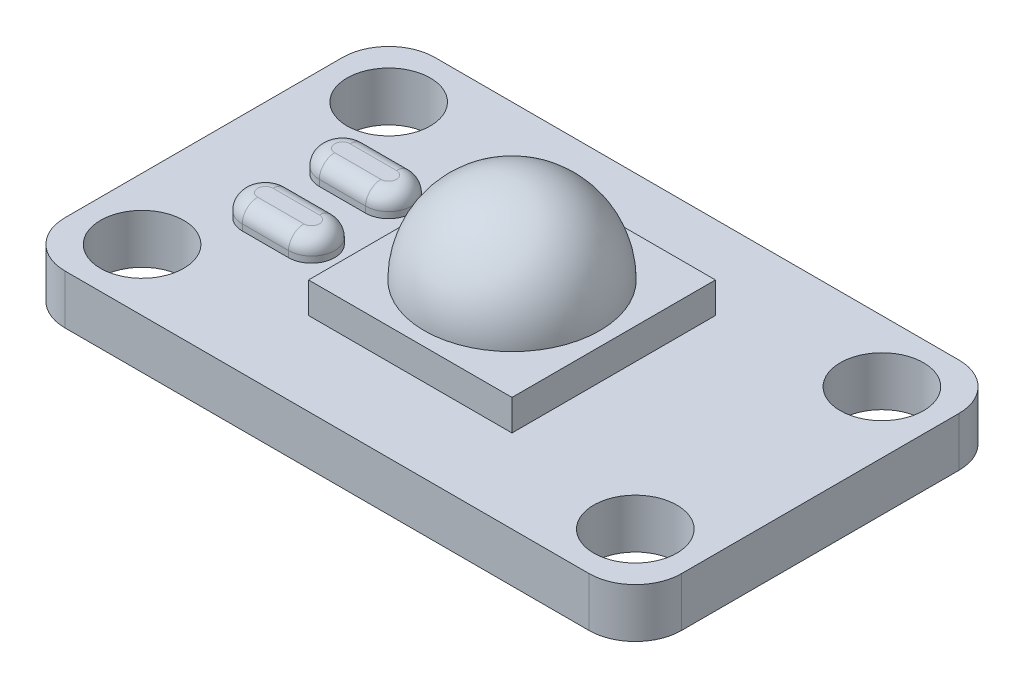
SolidWorks part; units mm, degrees
ref_plane "前视基准面" through (0, 0, 0) normal (0, 0, 1) x (1, 0, 0)
ref_plane "上视基准面" through (0, 0, 0) normal (0, 1, 0) x (1, 0, 0)
ref_plane "右视基准面" through (0, 0, 0) normal (1, 0, 0) x (0, 0, -1)
sketch "铝基板外型" plane through (0, 0, 0) normal (0, 1, 0) x (1, 0, 0)
  line L1 (-8.5, -6) -> (8.5, -6)
  line L2 (-10, -4.5) -> (-10, 4.5)
  line L3 (-8.5, 6) -> (8.5, 6)
  line L4 (10, -4.5) -> (10, 4.5)
  line L5 (-10, -6) -> (10, 6) construction
  line L6 (-10, 6) -> (10, -6) construction
  arc A0 (-8.5, -6) -> (-10, -4.5) centre (-8.5, -4.5) cw
  arc A1 (8.5, -6) -> (10, -4.5) centre (8.5, -4.5) ccw
  arc A2 (8.5, 6) -> (10, 4.5) centre (8.5, 4.5) cw
  arc A3 (-10, 4.5) -> (-8.5, 6) centre (-8.5, 4.5) cw
  point P0 (0, 0)
  dimension "D1" = 1.5
  dimension "D2" = 20
  dimension "D3" = 12
extrude "铝基板" add sketch "铝基板外型" along normal blind 1.6
sketch "草图7" plane through (0, 0, 0) normal (0, 1, 0) x (1, 0, 0)
  line L1 (-8, -4) -> (8, -4) construction
  line L2 (-8, -4) -> (-8, 4) construction
  line L3 (-8, 4) -> (8, 4) construction
  line L4 (8, -4) -> (8, 4) construction
  line L5 (-8, -4) -> (8, 4) construction
  line L6 (-8, 4) -> (8, -4) construction
  circle A0 centre (-8, -4) radius 1.35
  circle A1 centre (8, -4) radius 1.35
  circle A2 centre (8, 4) radius 1.35
  circle A3 centre (-8, 4) radius 1.35
  point P0 (0, 0)
  dimension "D3" = 2.7
  dimension "D1" = 8
  dimension "D2" = 16
extrude "螺丝孔" cut sketch "草图7" along normal through all
sketch "？？？" plane through (0, 1.6, 0) normal (0, 1, 0) x (1, 0, 0)
  line L1 (-3.3, 3.3) -> (3.3, 3.3)
  line L2 (-3.3, 3.3) -> (-3.3, -3.3)
  line L3 (-3.3, -3.3) -> (3.3, -3.3)
  line L4 (3.3, 3.3) -> (3.3, -3.3)
  line L5 (-3.3, 3.3) -> (3.3, -3.3) construction
  line L6 (-3.3, -3.3) -> (3.3, 3.3) construction
  point P0 (0, 0)
  dimension "D1" = 6.6
extrude "灯珠板" add sketch "？？？" along normal blind 1 separate body
sketch "灯珠旋转基础" plane through (0, 0, 0) normal (0, 0, 1) x (1, 0, 0)
  line L0 (0, 2.6) -> (2.85, 2.6)
  line L1 (0, 2.6) -> (0, 5.45)
  line L2 (-3.3, 2.6) -> (3.3, 2.6) construction
  arc A0 (0, 5.45) -> (2.85, 2.6) centre (0, 2.6) cw
  dimension "D1" = 2.85
revolve "灯珠" add sketch "灯珠旋转基础" angle 360 about L1
sketch "焊盘" plane through (0, 1.6, 0) normal (0, 1, 0) x (1, 0, 0)
  line L0 (-6.75, 1.25) -> (-5.25, 1.25) construction
  line L1 (-6.75, 2) -> (-5.25, 2)
  line L2 (-6.75, 0.5) -> (-5.25, 0.5)
  line L3 (-6.75, -1.25) -> (-5.25, -1.25) construction
  line L4 (-6.75, -0.5) -> (-5.25, -0.5)
  line L5 (-6.75, -2) -> (-5.25, -2)
  line L6 (-12.3939, 0) -> (49987.6061, 0) construction
  line L7 (-8.5, -6) -> (8.5, -6) construction
  line L8 (-10, 4.5) -> (-10, -4.5) construction
  arc A0 (-6.75, 2) -> (-6.75, 0.5) centre (-6.75, 1.25) ccw
  arc A1 (-5.25, 0.5) -> (-5.25, 2) centre (-5.25, 1.25) ccw
  arc A2 (-6.75, -0.5) -> (-6.75, -2) centre (-6.75, -1.25) ccw
  arc A3 (-5.25, -2) -> (-5.25, -0.5) centre (-5.25, -1.25) ccw
  point P2 (-6, 1.25)
  point P7 (-6, -1.25)
  dimension "D1" = 0.75
  dimension "D2" = 1.5
  dimension "D3" = 4.75
  dimension "D4" = 4
extrude "焊点基础外型" add sketch "焊盘" along normal blind 0.7 separate body
fillet "焊点1" radius 0.5 4 edges at (-6, 2.3, -2) (-4.5, 2.3, -1.25) (-6, 2.3, -0.5) (-7.5, 2.3, -1.25)
fillet "焊点2" radius 0.5 4 edges at (-6, 2.3, 2) (-7.5, 2.3, 1.25) (-6, 2.3, 0.5) (-4.5, 2.3, 1.25)
